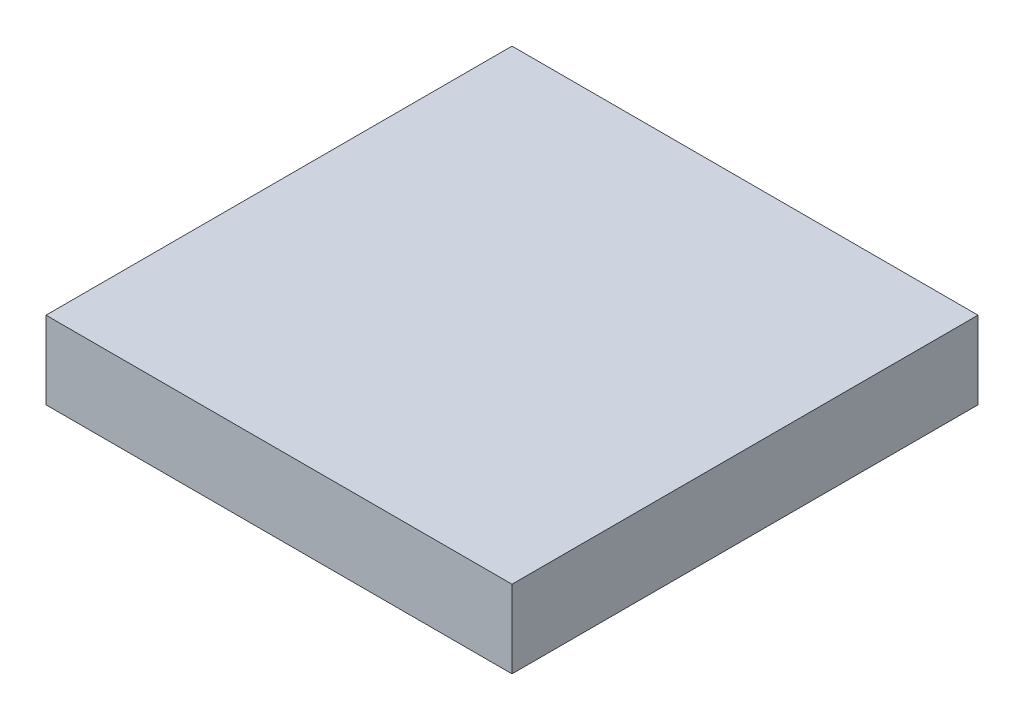
from build123d import *

# Parameters (mm, degrees)
SKETCH1_W           = 120
SKETCH1_H           = 120
BOSS_EXTRUDE1_DEPTH = 20


with BuildPart() as part:
    # Sketch1 → Boss-Extrude1 (new body)
    with BuildSketch(Plane(origin=(0, 0, 0), x_dir=(1, 0, 0), z_dir=(0, 1, 0))):
        Rectangle(SKETCH1_W, SKETCH1_H)
    extrude(amount=BOSS_EXTRUDE1_DEPTH)


solid = part.part
